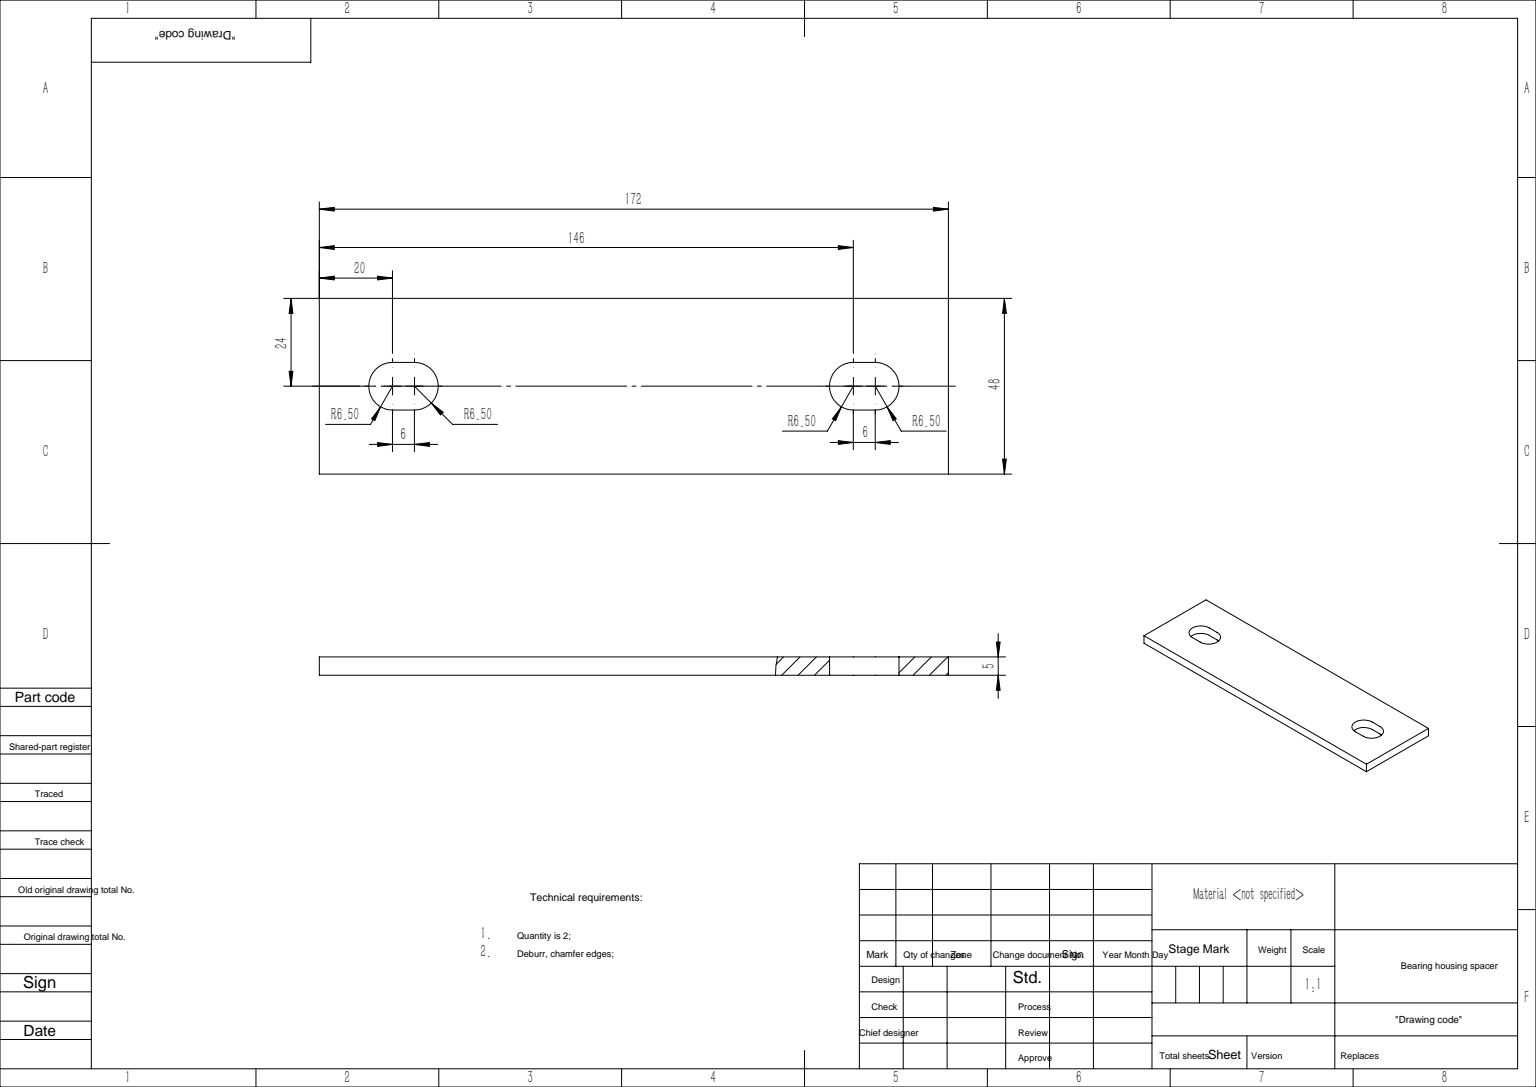
SolidWorks part; units mm, degrees
ref_plane "前视基准面" through (0, 0, 0) normal (0, 0, 1) x (1, 0, 0)
ref_plane "上视基准面" through (0, 0, 0) normal (0, 1, 0) x (1, 0, 0)
ref_plane "右视基准面" through (0, 0, 0) normal (1, 0, 0) x (0, 0, -1)
sketch "草图1" plane through (0, 0, 0) normal (0, 1, 0) x (1, 0, 0)
  line L1 (-86, -24) -> (86, -24)
  line L2 (-86, -24) -> (-86, 24)
  line L3 (-86, 24) -> (86, 24)
  line L4 (86, -24) -> (86, 24)
  line L5 (-86, -24) -> (86, 24) construction
  line L6 (-86, 24) -> (86, -24) construction
  point P0 (0, 0)
  dimension "D1" = 172
  dimension "D2" = 48
extrude "凸台-拉伸1" add sketch "草图1" along normal blind 5
sketch "草图2" plane through (0, 5, 0) normal (0, 1, 0) x (1, 0, 0)
  line L0 (66, -6.5) -> (60, -6.5) construction
  line L1 (60, 6.5) -> (66, 6.5) construction
  line L2 (-66, 6.5) -> (-60, 6.5) construction
  line L3 (-60, -6.5) -> (-66, -6.5) construction
  line L4 (66, -6.5) -> (60, -6.5)
  line L5 (60, 6.5) -> (66, 6.5)
  line L6 (-66, 6.5) -> (-60, 6.5)
  line L7 (-60, -6.5) -> (-66, -6.5)
  arc A0 (66, -6.5) -> (66, 6.5) centre (66, 0) ccw construction
  arc A1 (60, 6.5) -> (60, -6.5) centre (60, 0) ccw construction
  arc A2 (-60, -6.5) -> (-60, 6.5) centre (-60, 0) ccw construction
  arc A3 (-66, 6.5) -> (-66, -6.5) centre (-66, 0) ccw construction
  arc A4 (66, -6.5) -> (66, 6.5) centre (66, 0) ccw
  arc A5 (60, 6.5) -> (60, -6.5) centre (60, 0) ccw
  arc A6 (-60, -6.5) -> (-60, 6.5) centre (-60, 0) ccw
  arc A7 (-66, 6.5) -> (-66, -6.5) centre (-66, 0) ccw
extrude "切除-拉伸1" cut sketch "草图2" against normal through all
